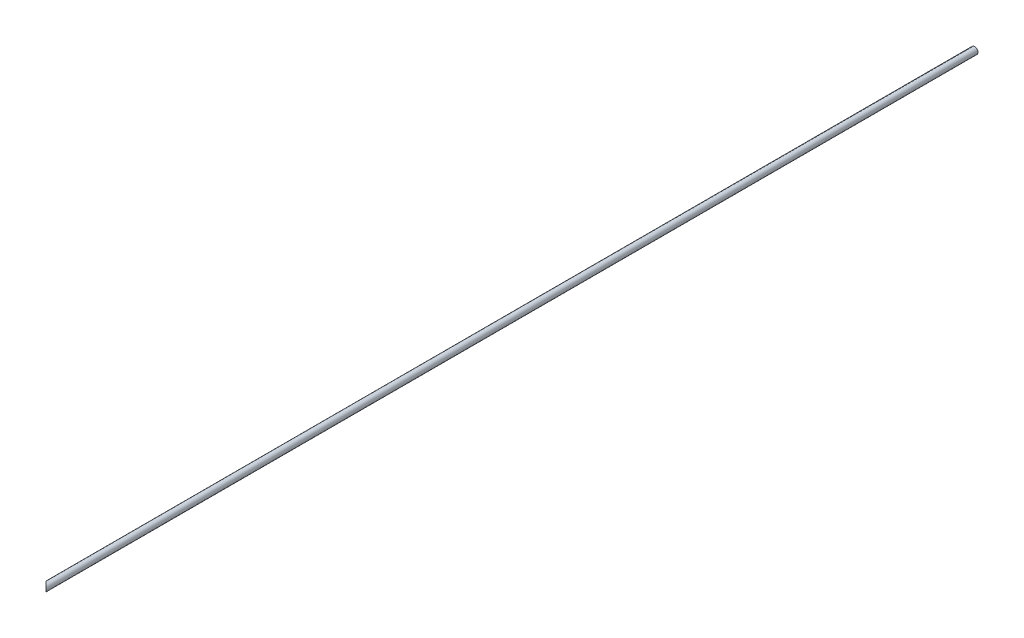
SolidWorks part; units mm, degrees
material "SWM-B"
ref_plane "Front Plane" through (0, 0, 0) normal (0, 0, 1) x (1, 0, 0)
ref_plane "Top Plane" through (0, 0, 0) normal (0, 1, 0) x (1, 0, 0)
ref_plane "Right Plane" through (0, 0, 0) normal (1, 0, 0) x (0, 0, -1)
sketch "Sketch1" plane through (0, 0, 0) normal (0, 0, 1) x (1, 0, 0)
  circle A0 centre (0, 0) radius 3
  dimension "D1" = 6
extrude "Boss-Extrude1" add sketch "Sketch1" along normal blind 832.8
sketch "Sketch2" plane through (0, 0, 0) normal (0, 1, 0) x (1, 0, 0)
  line L0 (3, -832.8) -> (-3, -826.8)
  line L1 (-3, 0) -> (-3, -832.8) construction
  line L2 (-3, -826.8) -> (-3, -832.8)
  line L3 (-3, -832.8) -> (3, -832.8)
  dimension "D1" = 6
extrude "Cut-Extrude1" cut sketch "Sketch2" against normal through all both and the other way through all
